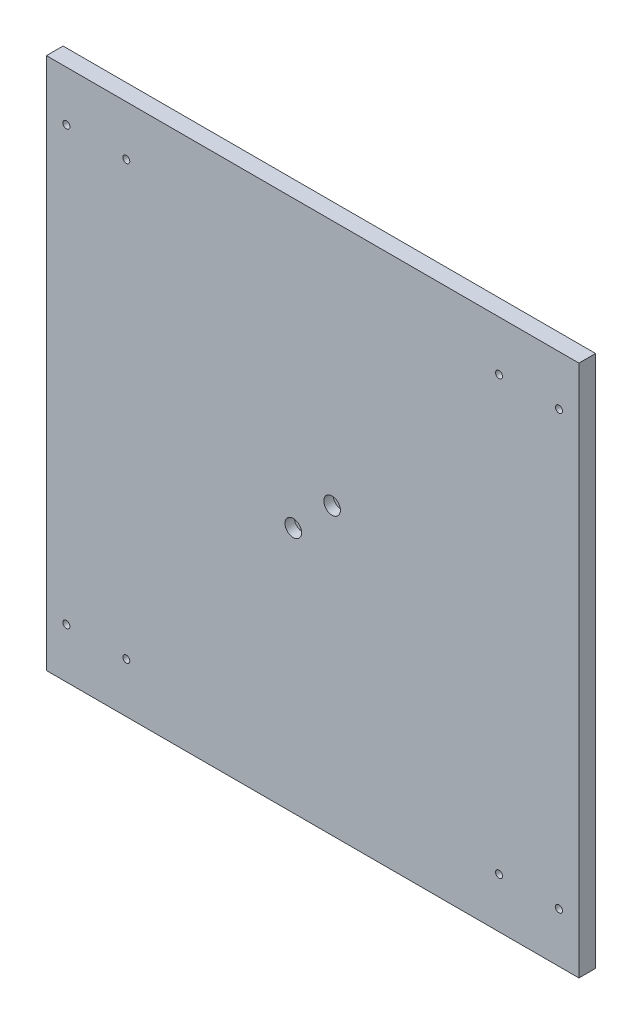
from build123d import *

# Parameters (mm, degrees)
SKETCH_1_W                = 320
SKETCH_1_H                = 320
EXTRUDE_1_DEPTH           = 10
HOLE_WIZARD_1_D           = 5.5
HOLE_WIZARD_1_DEPTH       = 10
HOLE_WIZARD_1_CBORE_D     = 10
HOLE_WIZARD_1_CBORE_DEPTH = 5.7
HOLE_WIZARD_1_TIP         = 1.652366702
HOLE_WIZARD_M5_1_D        = 4.2
MIRROR_2_COPY_1_D         = 4.2


with BuildPart() as part:
    # 草图1 → 凸台-拉伸1 (new body)
    with BuildSketch(Plane.XY):
        Rectangle(SKETCH_1_W, SKETCH_1_H)
    extrude(amount=EXTRUDE_1_DEPTH)

    # 打孔尺寸(%根据)内六角圆柱头螺钉的类型1
    with Locations(Plane.XY.offset(10)):
        with Locations((-11.66726189, -11.66726189), (11.66726189, 11.66726189)):
            CounterBoreHole(HOLE_WIZARD_1_D / 2, HOLE_WIZARD_1_CBORE_D / 2, HOLE_WIZARD_1_CBORE_DEPTH, depth=HOLE_WIZARD_1_DEPTH)
            with Locations((0, 0, -(HOLE_WIZARD_1_DEPTH + HOLE_WIZARD_1_TIP / 2))):  # 118° drill point
                Cone(0, HOLE_WIZARD_1_D / 2, HOLE_WIZARD_1_TIP, mode=Mode.SUBTRACT)

    # M5 螺纹孔1 (through all)
    with Locations(Plane(origin=(0, 0, 0), x_dir=(-1, 0, 0), z_dir=(0, 0, -1))):
        with Locations((-148, 130), (-112, 130)):
            hole_wizard_m5_1 = Hole(HOLE_WIZARD_M5_1_D / 2)

    # 镜向1: M5 螺纹孔1 across plane
    add(hole_wizard_m5_1.mirror(Plane.ZX), mode=Mode.SUBTRACT)

    # 镜向2: M5 螺纹孔1 across plane
    add(hole_wizard_m5_1.mirror(Plane(origin=(0, 0, 0), x_dir=(0, 0, 1), z_dir=(1, 0, 0))), mode=Mode.SUBTRACT)

    # 镜向2 copy 1 (through all)
    with Locations(Plane(origin=(0, 0, 0), x_dir=(1, 0, 0), z_dir=(0, 0, -1))):
        with Locations((-148, 130), (-112, 130)):
            Hole(MIRROR_2_COPY_1_D / 2)


solid = part.part
